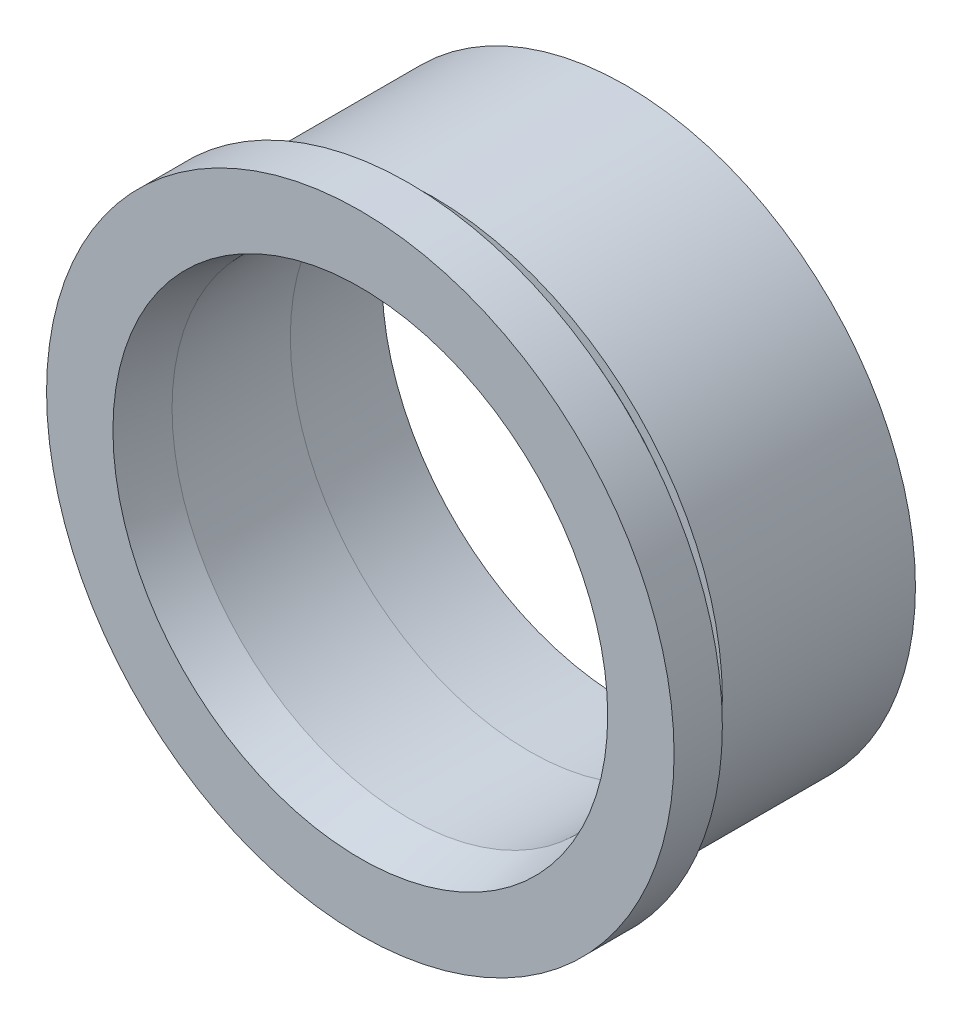
SolidWorks part; units mm, degrees
ref_plane "Front Plane" through (0, 0, 0) normal (0, 0, 1) x (1, 0, 0)
ref_plane "Top Plane" through (0, 0, 0) normal (0, 1, 0) x (1, 0, 0)
ref_plane "Right Plane" through (0, 0, 0) normal (1, 0, 0) x (0, 0, -1)
ref_plane "Plane1" through (0, 234.744, 0) normal (0, 1, 0) x (1, 0, 0)
sketch "Sketch1" plane through (0, 234.744, 0) normal (0, 1, 0) x (1, 0, 0)
  line L0 (586.2306, 1054.693) -> (579.2306, 1054.693)
  line L1 (579.2306, 1054.693) -> (579.2306, 1059.693)
  line L2 (579.2306, 1059.693) -> (581.2306, 1059.693)
  line L3 (581.2306, 1059.693) -> (581.2306, 1099.693)
  line L4 (581.2306, 1099.693) -> (571.7306, 1099.693)
  line L5 (571.7306, 1099.693) -> (570.7306, 1079.693)
  line L6 (570.7306, 1079.693) -> (570.2306, 1054.693)
  line L7 (570.2306, 1054.693) -> (572.4806, 1044.693)
  line L8 (572.4806, 1044.693) -> (586.2306, 1044.693)
  line L9 (586.2306, 1044.693) -> (586.2306, 1054.693)
  line L10 (521.2306, 1099.693) -> (521.2306, 1044.693) construction
  dimension "D1" = 49
  dimension "D2" = 49.5
  dimension "D3" = 50.5
  dimension "D4" = 51.25
  dimension "D5" = 58
  dimension "D6" = 60
  dimension "D7" = 65
  dimension "D8" = 10
  dimension "D9" = 15
  dimension "D10" = 35
  dimension "D11" = 55
revolve "Revolve1" add sketch "Sketch1" angle 360 about L10
